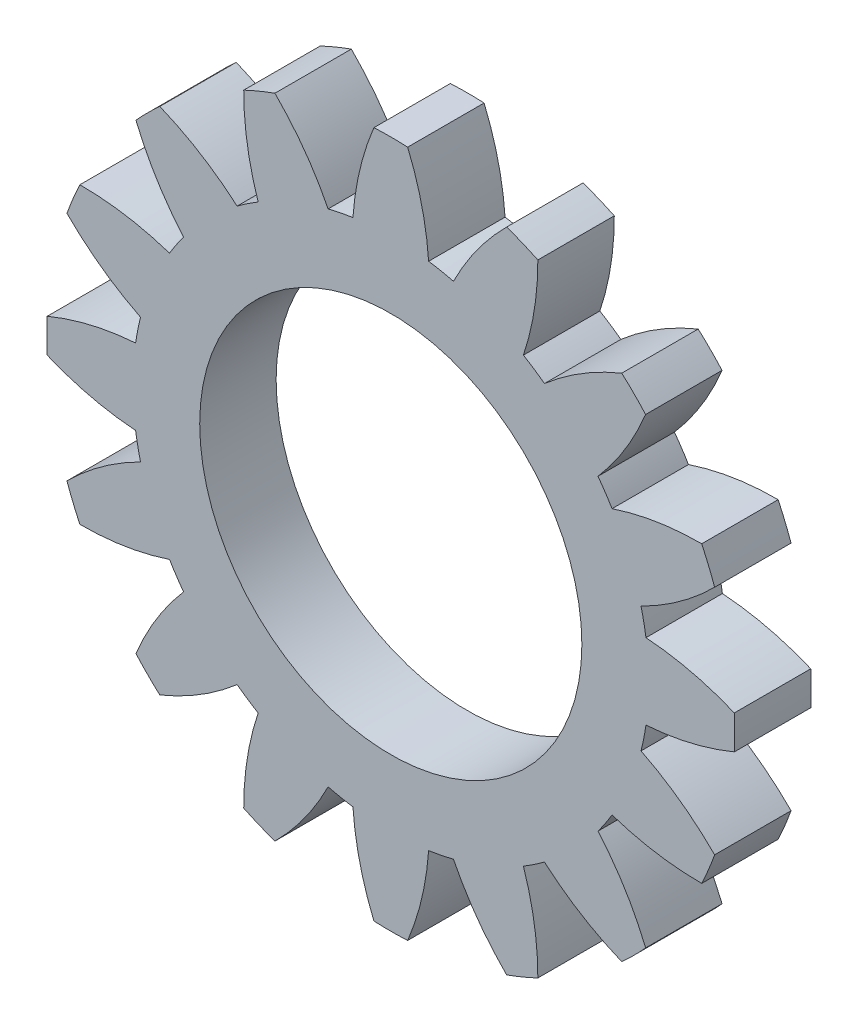
from build123d import *

# Parameters (mm, degrees)
SKETCH1_R           = 10
BOSS_EXTRUDE1_DEPTH = 4


with BuildPart() as part:
    # Sketch1 → Boss-Extrude1 (new body)
    with BuildSketch(Plane(origin=(0, 0, 0), x_dir=(-1, 0, 0), z_dir=(0, 0, -1))):
        with BuildLine():
            ThreePointArc((6.940387047, 11.579336235), (7.509222961, 13.894810592), (7.695991682, 16.271807276))
            ThreePointArc((7.695991682, 16.271807276), (6.888301783, 16.629831585), (6.064017361, 16.947793173))
            ThreePointArc((6.064017361, 16.947793173), (4.515292316, 15.13493727), (3.280232429, 13.095421918))
            ThreePointArc((3.280232429, 13.095421918), (2.633719347, 13.240601285), (1.980861405, 13.353882885))
            ThreePointArc((1.980861405, 13.353882885), (1.620303589, 15.710786331), (0.883218138, 17.978318212))
            ThreePointArc((0.883218138, 17.978318212), (0, 18), (-0.883218138, 17.978318212))
            ThreePointArc((-0.883218138, 17.978318212), (-1.620303589, 15.710786331), (-1.980861405, 13.353882885))
            ThreePointArc((-1.980861405, 13.353882885), (-2.633719347, 13.240601285), (-3.280232429, 13.095421918))
            ThreePointArc((-3.280232429, 13.095421918), (-4.515292316, 15.13493727), (-6.064017361, 16.947793173))
            ThreePointArc((-6.064017361, 16.947793173), (-6.888301783, 16.629831585), (-7.695991682, 16.271807276))
            ThreePointArc((-7.695991682, 16.271807276), (-7.509222961, 13.894810592), (-6.940387047, 11.579336235))
            ThreePointArc((-6.940387047, 11.579336235), (-7.500198146, 11.224839766), (-8.041940611, 10.843301675))
            ThreePointArc((-8.041940611, 10.843301675), (-9.963475897, 12.254931208), (-12.088061187, 13.337120256))
            ThreePointArc((-12.088061187, 13.337120256), (-12.727922061, 12.727922061), (-13.337120256, 12.088061187))
            ThreePointArc((-13.337120256, 12.088061187), (-12.254931208, 9.963475897), (-10.843301675, 8.041940611))
            ThreePointArc((-10.843301675, 8.041940611), (-11.224839766, 7.500198146), (-11.579336235, 6.940387047))
            ThreePointArc((-11.579336235, 6.940387047), (-13.894810592, 7.509222961), (-16.271807276, 7.695991682))
            ThreePointArc((-16.271807276, 7.695991682), (-16.629831585, 6.888301783), (-16.947793173, 6.064017361))
            ThreePointArc((-16.947793173, 6.064017361), (-15.13493727, 4.515292316), (-13.095421918, 3.280232429))
            ThreePointArc((-13.095421918, 3.280232429), (-13.240601285, 2.633719347), (-13.353882885, 1.980861405))
            ThreePointArc((-13.353882885, 1.980861405), (-15.710786331, 1.620303589), (-17.978318212, 0.883218138))
            ThreePointArc((-17.978318212, 0.883218138), (-18, 0), (-17.978318212, -0.883218138))
            ThreePointArc((-17.978318212, -0.883218138), (-15.710786331, -1.620303589), (-13.353882885, -1.980861405))
            ThreePointArc((-13.353882885, -1.980861405), (-13.240601285, -2.633719347), (-13.095421918, -3.280232429))
            ThreePointArc((-13.095421918, -3.280232429), (-15.13493727, -4.515292316), (-16.947793173, -6.064017361))
            ThreePointArc((-16.947793173, -6.064017361), (-16.629831585, -6.888301783), (-16.271807276, -7.695991682))
            ThreePointArc((-16.271807276, -7.695991682), (-13.894810592, -7.509222961), (-11.579336235, -6.940387047))
            ThreePointArc((-11.579336235, -6.940387047), (-11.224839766, -7.500198146), (-10.843301675, -8.041940611))
            ThreePointArc((-10.843301675, -8.041940611), (-12.254931208, -9.963475897), (-13.337120256, -12.088061187))
            ThreePointArc((-13.337120256, -12.088061187), (-12.727922061, -12.727922061), (-12.088061187, -13.337120256))
            ThreePointArc((-12.088061187, -13.337120256), (-9.963475897, -12.254931208), (-8.041940611, -10.843301675))
            ThreePointArc((-8.041940611, -10.843301675), (-7.500198146, -11.224839766), (-6.940387047, -11.579336235))
            ThreePointArc((-6.940387047, -11.579336235), (-7.509222961, -13.894810592), (-7.695991682, -16.271807276))
            ThreePointArc((-7.695991682, -16.271807276), (-6.888301783, -16.629831585), (-6.064017361, -16.947793173))
            ThreePointArc((-6.064017361, -16.947793173), (-4.515292316, -15.13493727), (-3.280232429, -13.095421918))
            ThreePointArc((-3.280232429, -13.095421918), (-2.633719347, -13.240601285), (-1.980861405, -13.353882885))
            ThreePointArc((-1.980861405, -13.353882885), (-1.620303589, -15.710786331), (-0.883218138, -17.978318212))
            ThreePointArc((-0.883218138, -17.978318212), (0, -18), (0.883218138, -17.978318212))
            ThreePointArc((0.883218138, -17.978318212), (1.620303589, -15.710786331), (1.980861405, -13.353882885))
            ThreePointArc((1.980861405, -13.353882885), (2.633719347, -13.240601285), (3.280232429, -13.095421918))
            ThreePointArc((3.280232429, -13.095421918), (4.515292316, -15.13493727), (6.064017361, -16.947793173))
            ThreePointArc((6.064017361, -16.947793173), (6.888301783, -16.629831585), (7.695991682, -16.271807276))
            ThreePointArc((7.695991682, -16.271807276), (7.509222961, -13.894810592), (6.940387047, -11.579336235))
            ThreePointArc((6.940387047, -11.579336235), (7.500198146, -11.224839766), (8.041940611, -10.843301675))
            ThreePointArc((8.041940611, -10.843301675), (9.963475897, -12.254931208), (12.088061187, -13.337120256))
            ThreePointArc((12.088061187, -13.337120256), (12.727922061, -12.727922061), (13.337120256, -12.088061187))
            ThreePointArc((13.337120256, -12.088061187), (12.254931208, -9.963475897), (10.843301675, -8.041940611))
            ThreePointArc((10.843301675, -8.041940611), (11.224839766, -7.500198146), (11.579336235, -6.940387047))
            ThreePointArc((11.579336235, -6.940387047), (13.894810592, -7.509222961), (16.271807276, -7.695991682))
            ThreePointArc((16.271807276, -7.695991682), (16.629831585, -6.888301783), (16.947793173, -6.064017361))
            ThreePointArc((16.947793173, -6.064017361), (15.13493727, -4.515292316), (13.095421918, -3.280232429))
            ThreePointArc((13.095421918, -3.280232429), (13.240601285, -2.633719347), (13.353882885, -1.980861405))
            ThreePointArc((13.353882885, -1.980861405), (15.710786331, -1.620303589), (17.978318212, -0.883218138))
            ThreePointArc((17.978318212, -0.883218138), (18, 0), (17.978318212, 0.883218138))
            ThreePointArc((17.978318212, 0.883218138), (15.710786331, 1.620303589), (13.353882885, 1.980861405))
            ThreePointArc((13.353882885, 1.980861405), (13.240601285, 2.633719347), (13.095421918, 3.280232429))
            ThreePointArc((13.095421918, 3.280232429), (15.13493727, 4.515292316), (16.947793173, 6.064017361))
            ThreePointArc((16.947793173, 6.064017361), (16.629831585, 6.888301783), (16.271807276, 7.695991682))
            ThreePointArc((16.271807276, 7.695991682), (13.894810592, 7.509222961), (11.579336235, 6.940387047))
            ThreePointArc((11.579336235, 6.940387047), (11.224839766, 7.500198146), (10.843301675, 8.041940611))
            ThreePointArc((10.843301675, 8.041940611), (12.254931208, 9.963475897), (13.337120256, 12.088061187))
            ThreePointArc((13.337120256, 12.088061187), (12.727922061, 12.727922061), (12.088061187, 13.337120256))
            ThreePointArc((12.088061187, 13.337120256), (9.963475897, 12.254931208), (8.041940611, 10.843301675))
            ThreePointArc((8.041940611, 10.843301675), (7.500198146, 11.224839766), (6.940387047, 11.579336235))
        make_face()
        with Locations(Location((0, 0, 0), (0, 0, 180))):
            Circle(SKETCH1_R, mode=Mode.SUBTRACT)
    extrude(amount=-BOSS_EXTRUDE1_DEPTH)


solid = part.part
